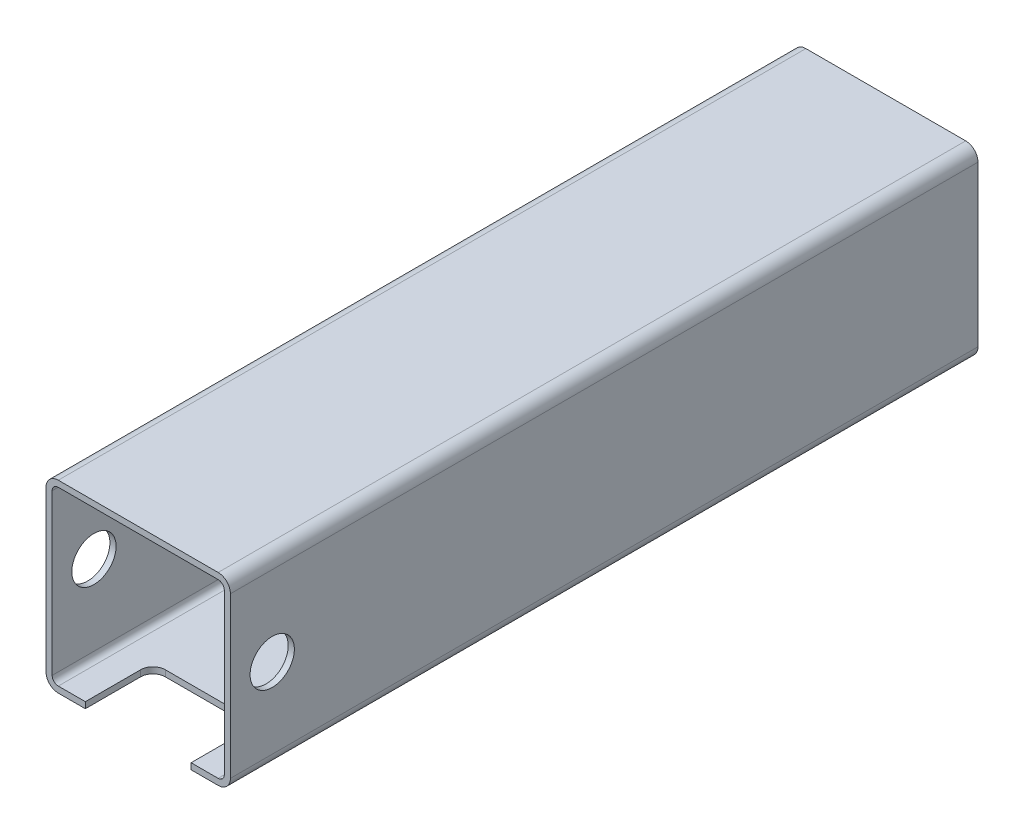
from build123d import *

# Parameters (mm, degrees)
SKETCH1_W           = 150
SKETCH1_H           = 150
SKETCH1_W_2         = 140
SKETCH1_H_2         = 140
BOSS_EXTRUDE1_DEPTH = 608
FILLET1_R           = 10
FILLET2_R           = 5
SKETCH2_R           = 18
CUT_EXTRUDE1_DEPTH  = 644.944096953
SKETCH3_W           = 86
SKETCH3_H           = 55
CUT_EXTRUDE2_DEPTH  = 10
FILLET3_R           = 10


with BuildPart() as part:
    # Sketch1 → Boss-Extrude1 (new body)
    with BuildSketch(Plane.XY):
        with Locations((75, 75)):
            Rectangle(SKETCH1_W, SKETCH1_H)
        with Locations((75, 75)):
            Rectangle(SKETCH1_W_2, SKETCH1_H_2, mode=Mode.SUBTRACT)
    extrude(amount=BOSS_EXTRUDE1_DEPTH)

    # Fillet1
    fillet1_edges = [part.edges().sort_by_distance(p)[0] for p in [
        (0, 150, 304),
        (150, 150, 304),
        (150, 0, 304),
        (0, 0, 304),
    ]]
    fillet(fillet1_edges, radius=FILLET1_R)

    # Fillet2
    fillet2_edges = [part.edges().sort_by_distance(p)[0] for p in [
        (5, 145, 304),
        (5, 5, 304),
        (145, 5, 304),
        (145, 145, 304),
    ]]
    fillet(fillet2_edges, radius=FILLET2_R)

    # Sketch2 → Cut-Extrude1 (cut, through all)
    with BuildSketch(Plane.ZY):
        with Locations((574, 75)):
            Circle(SKETCH2_R)
    extrude(amount=-CUT_EXTRUDE1_DEPTH, mode=Mode.SUBTRACT)

    # Sketch3 → Cut-Extrude2 (cut)
    with BuildSketch(Plane.XZ):
        with Locations((75, 580.5)):
            Rectangle(SKETCH3_W, SKETCH3_H)
    extrude(amount=-CUT_EXTRUDE2_DEPTH, mode=Mode.SUBTRACT)

    # Fillet3
    fillet3_edges = [part.edges().sort_by_distance(p)[0] for p in [
        (32, 2.5, 553),
        (118, 2.5, 553),
    ]]
    fillet(fillet3_edges, radius=FILLET3_R)


solid = part.part
